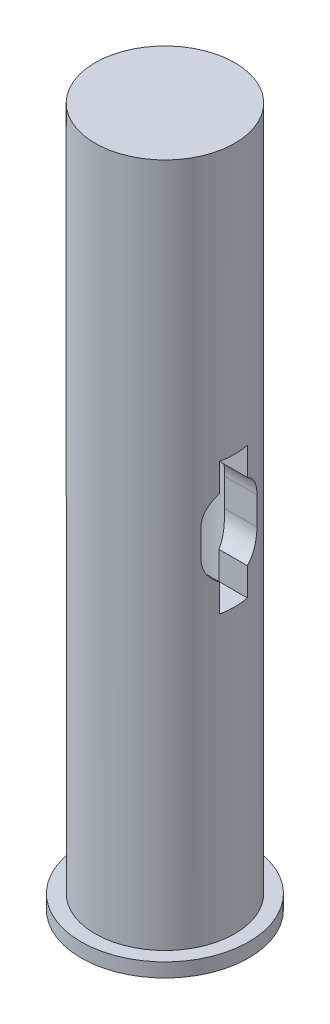
SolidWorks part; units mm, degrees
ref_plane "Front Plane" through (0, 0, 0) normal (0, 0, 1) x (1, 0, 0)
ref_plane "Top Plane" through (0, 0, 0) normal (0, 1, 0) x (1, 0, 0)
ref_plane "Right Plane" through (0, 0, 0) normal (1, 0, 0) x (0, 0, -1)
other "Configuration Table"
sketch "Sketch3" plane through (0, 0, 0) normal (0, 0, 1) x (1, 0, 0)
  line L0 (3.025, 0) -> (3.025, 32.1)
  line L1 (3.025, 32.1) -> (0, 32.1)
  line L2 (0, 32.1) -> (0, 50)
  line L3 (0, 50) -> (5, 50)
  line L4 (5, 50) -> (5, 0)
  line L5 (5, 0) -> (3.025, 0)
  line L6 (0, -0.7297) -> (0, 3.7297) construction
  line L7 (-4.8288, 0) -> (11.2175, 0) construction
  dimension "D1" = 10
  dimension "D2" = 6.05
  dimension "D3" = 50
  dimension "D4" = 32.1
revolve "Revolve1" add sketch "Sketch3" angle 360 about L6
ref_plane "Plane1" through (5, 0, 0) normal (1, 0, 0) x (0, 0, -1)
sketch "Sketch6" plane through (5, 0, 0) normal (1, 0, 0) x (0, 0, -1)
  line L0 (0, -4.0653) -> (0, 40.3862) construction
  line L1 (0, 27) -> (0, 25) construction
  line L2 (2, 27) -> (2, 25)
  line L3 (-2, 27) -> (-2, 25)
  arc A1 (2, 27) -> (-2, 27) centre (0, 27) ccw
  arc A2 (-2, 25) -> (2, 25) centre (0, 25) ccw
  point P5 (0, 26)
  dimension "D1" = 2
  dimension "D3" = 25
  dimension "D2" = 2
extrude "Cut-Extrude1" cut sketch "Sketch6" against normal through all
sketch "Sketch9" plane through (0, 0, 0) normal (0, 1, 0) x (1, 0, 0)
  circle A0 centre (0, 0) radius 6
  circle A1 centre (0, 0) radius 3
  dimension "D1" = 12
  dimension "D2" = 6
extrude "Boss-Extrude3" add sketch "Sketch9" along normal blind 1
sketch "Sketch11" plane through (5, 0, 0) normal (1, 0, 0) x (0, 0, -1)
  line L0 (0, 23) -> (0, 29) construction
  line L1 (-2, 26) -> (2, 26) construction
  line L2 (-2, 27) -> (-2, 25) construction
  line L3 (2, 25) -> (2, 27) construction
  line L4 (-1, 23.2679) -> (-1, 21.2679)
  line L5 (-1, 21.2679) -> (1, 21.2679)
  line L6 (1, 21.2679) -> (1, 23.2679)
  line L7 (-1, 28.7321) -> (-1, 30.7321)
  line L8 (-1, 30.7321) -> (1, 30.7321)
  line L9 (1, 30.7321) -> (1, 28.7321)
  line L10 (-1, 23.2679) -> (-1, 28.7321)
  line L11 (1, 28.7321) -> (1, 23.2679)
  arc A0 (-2, 25) -> (2, 25) centre (0, 25) ccw construction
  arc A1 (2, 27) -> (-2, 27) centre (0, 27) ccw construction
  arc A2 (-2, 25) -> (2, 25) centre (0, 25) ccw construction
  dimension "D1" = 2
  dimension "D2" = 2
  dimension "D3" = 2
  dimension "D4" = 2
extrude "Cut-Extrude2" cut sketch "Sketch11" against normal through all
